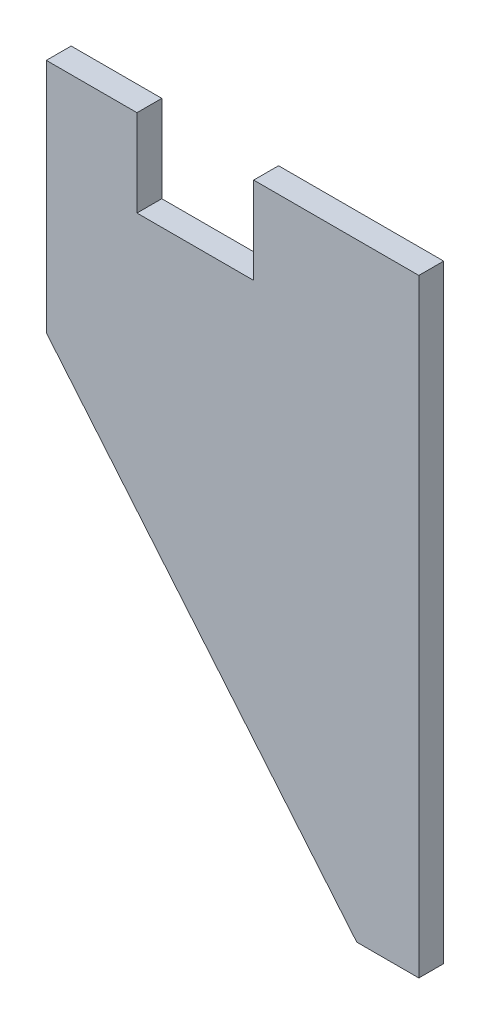
from build123d import *

# Parameters (mm, degrees)
BOSS_EXTRUDE1_DEPTH = 20


with BuildPart() as part:
    # Sketch1 → Boss-Extrude1 (new body)
    with BuildSketch(Plane.XY):
        Polygon((0, 0), (0, -490), (-50, -490), (-300, -190), (-300, 0), (-227, 0), (-227, -70), (-133, -70), (-133, 0), align=None)
    extrude(amount=BOSS_EXTRUDE1_DEPTH)


solid = part.part
